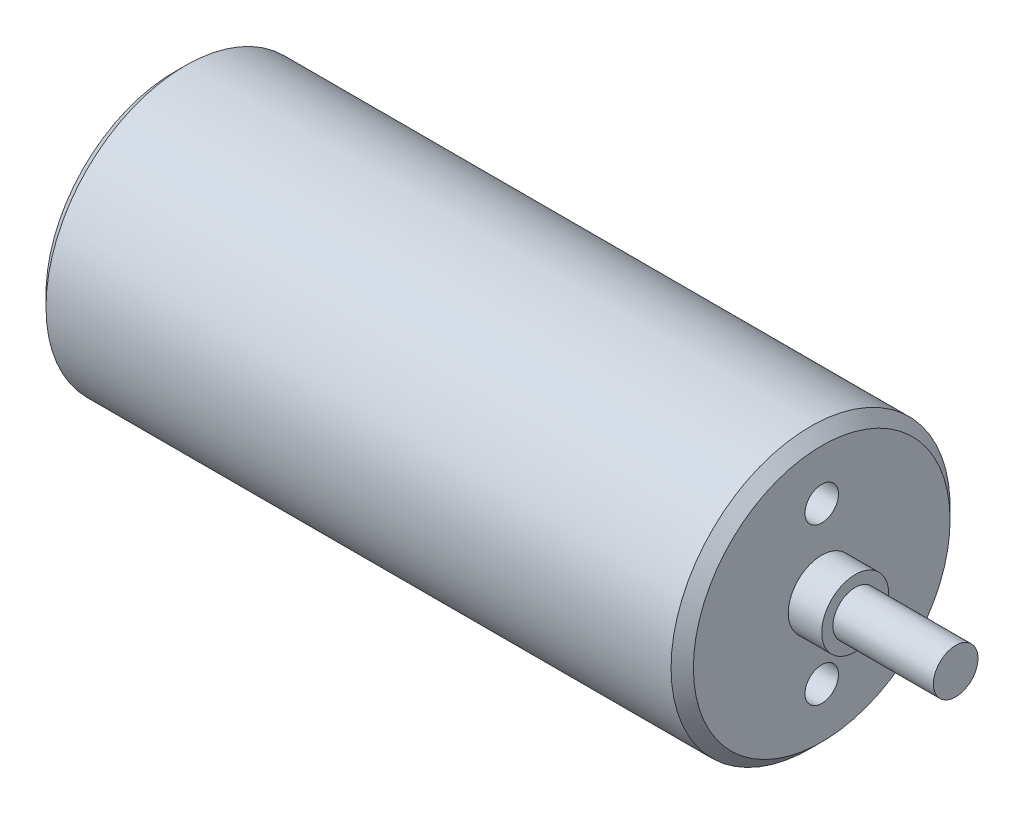
from build123d import *

# Parameters (mm, degrees)
SKETCH1_R           = 12.5
BOSS_EXTRUDE1_DEPTH = 58
SKETCH2_R           = 3
BOSS_EXTRUDE2_DEPTH = 3
SKETCH3_R           = 2
BOSS_EXTRUDE3_DEPTH = 9
SKETCH4_R           = 1.5
CUT_EXTRUDE1_DEPTH  = 6
CHAMFER1_SIZE       = 1
CHAMFER2_SIZE       = 1


with BuildPart() as part:
    # Sketch1 → Boss-Extrude1 (new body)
    with BuildSketch(Plane(origin=(0, 0, 0), x_dir=(0, 0, -1), z_dir=(1, 0, 0))):
        with Locations(Location((0, 0, 0), (0, 0, 180))):
            Circle(SKETCH1_R)
    extrude(amount=BOSS_EXTRUDE1_DEPTH)

    # Sketch2 → Boss-Extrude2 (add)
    with BuildSketch(Plane(origin=(58, 0, 0), x_dir=(0, 0, -1), z_dir=(1, 0, 0))):
        Circle(SKETCH2_R)
    extrude(amount=BOSS_EXTRUDE2_DEPTH)

    # Sketch3 → Boss-Extrude3 (add)
    with BuildSketch(Plane(origin=(61, 0, 0), x_dir=(0, 0, -1), z_dir=(1, 0, 0))):
        Circle(SKETCH3_R)
    extrude(amount=BOSS_EXTRUDE3_DEPTH)

    # Sketch4 → Cut-Extrude1 (cut)
    with BuildSketch(Plane(origin=(58, 0, 0), x_dir=(0, 0, -1), z_dir=(1, 0, 0))):
        with Locations((0, 7)):
            Circle(SKETCH4_R)
        with Locations(Location((0, -7, 0), (0, 0, 180))):
            Circle(SKETCH4_R)
    extrude(amount=-CUT_EXTRUDE1_DEPTH, mode=Mode.SUBTRACT)

    # Chamfer1
    chamfer1_edges = [part.edges().sort_by_distance(p)[0] for p in [
        (58, 0, -12.5),
    ]]
    chamfer(chamfer1_edges, length=CHAMFER1_SIZE)

    # Chamfer2
    chamfer2_edges = [part.edges().sort_by_distance(p)[0] for p in [
        (0, 0, -12.5),
    ]]
    chamfer(chamfer2_edges, length=CHAMFER2_SIZE)


solid = part.part
